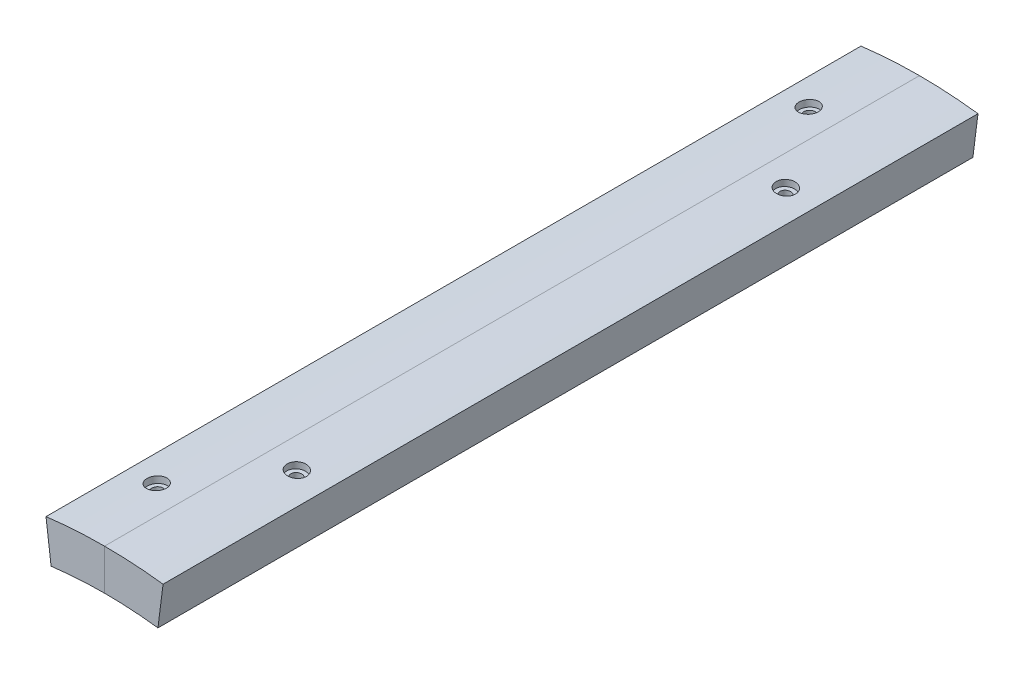
from build123d import *

# Parameters (mm, degrees)
BOSS_EXTRUDE1_DEPTH = 500
BOSS_EXTRUDE2_DEPTH = 500


with BuildPart() as part:
    # Sketch 1_3 → Boss-Extrude1 (new, symmetric)
    with BuildSketch(Plane.XY):
        with BuildLine():
            Line((-71.815942832, 568.481723853), (-65.549281154, 518.875988787))
            ThreePointArc((-65.549281154, 518.875988787), (-32.839441714, 521.967978968), (0, 523))
            Line((0, 523), (0, 573))
            ThreePointArc((0, 573), (-35.97896769, 571.869315389), (-71.815942832, 568.481723853))
        make_face()
    extrude(amount=BOSS_EXTRUDE1_DEPTH, both=True)

    # Sketch7 → CBORE for M12 Hex Head Bolt1 (revolve, cut)
    with BuildSketch(Plane(origin=(-35.97896769, 571.869315389, -400), x_dir=(-0.9980267284282717, -0.06279051952931308, 0), z_dir=(0, 0, 1))):
        Polygon((0, 0), (0, 55.14789445), (6.75, 55.14789445), (6.75, 7.95), (11.89, 7.95), (11.89, 0), align=None)
    cbore_for_m12_hex_head_bolt1 = revolve(axis=Axis((-36.377687489, 578.206785115, -400), (0.0627905195293131, -0.9980267284282717, 0)), mode=Mode.SUBTRACT)

    # Mirror2: CBORE for M12 Hex Head Bolt1 across plane
    add(cbore_for_m12_hex_head_bolt1.mirror(Plane.XY), mode=Mode.SUBTRACT)


with BuildPart() as body_2:
    # Sketch 1_3 2 → Boss-Extrude2 (new, symmetric)
    with BuildSketch(Plane.XY):
        with BuildLine():
            Line((0, 573), (0, 523))
            ThreePointArc((0, 523), (32.839441714, 521.967978968), (65.549281154, 518.875988787))
            Line((65.549281154, 518.875988787), (71.815942832, 568.481723853))
            ThreePointArc((71.815942832, 568.481723853), (35.97896769, 571.869315389), (0, 573))
        make_face()
    extrude(amount=BOSS_EXTRUDE2_DEPTH, both=True)

    # Sketch9 → CBORE for M12 Hex Head Bolt2 (revolve, cut)
    with BuildSketch(Plane(origin=(35.97896769, 571.869315389, -300), x_dir=(-0.9980267284282716, 0.06279051952931385, 0), z_dir=(0, 0, 1))):
        Polygon((0, 0), (0, 59.657254811), (6.75, 59.657254811), (6.75, 7.95), (11.89, 7.95), (11.89, 0), align=None)
    cbore_for_m12_hex_head_bolt2 = revolve(axis=Axis((36.377687489, 578.206785115, -300), (-0.0627905195293138, -0.9980267284282716, 0)), mode=Mode.SUBTRACT)

    # Mirror1: CBORE for M12 Hex Head Bolt2 across plane
    add(cbore_for_m12_hex_head_bolt2.mirror(Plane.XY), mode=Mode.SUBTRACT)


solid = Compound([part.part, body_2.part])
